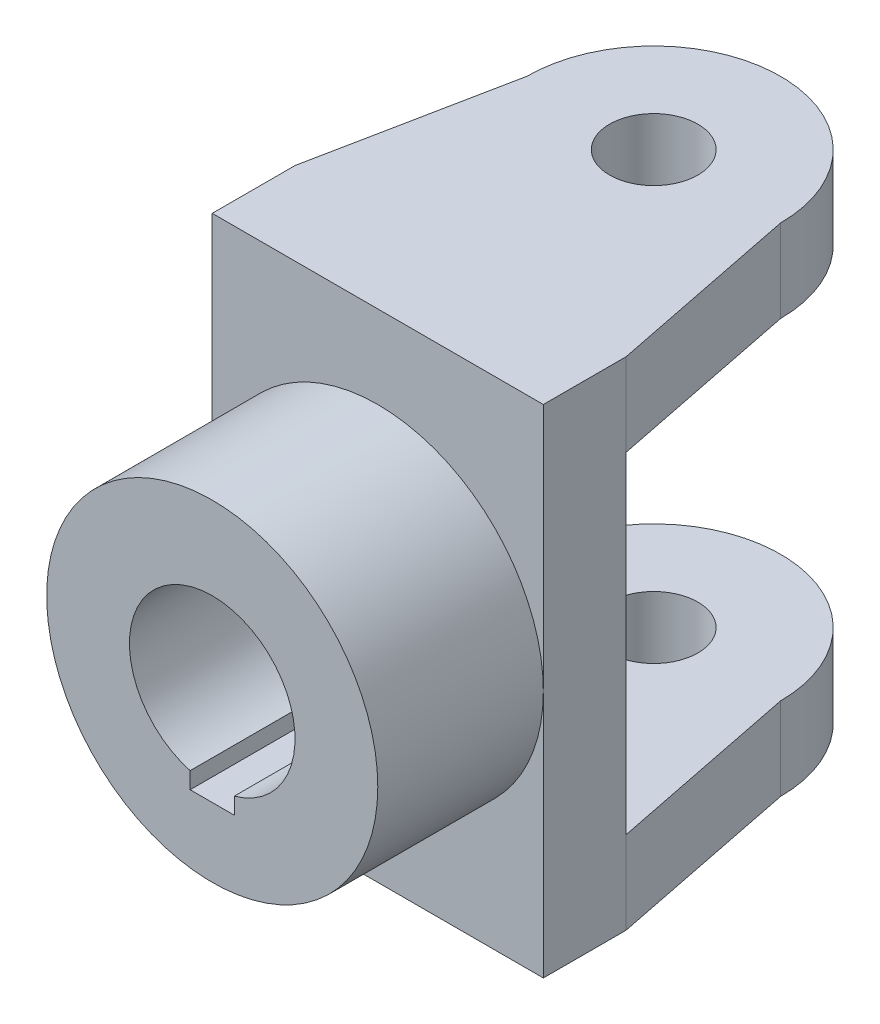
from build123d import *

# Parameters (mm, degrees)
SKETCH1_W           = 60
SKETCH1_H           = 90
BOSS_EXTRUDE1_DEPTH = 15
SKETCH2_R           = 8
BOSS_EXTRUDE2_DEPTH = 15
SKETCH3_R           = 30
BOSS_EXTRUDE3_DEPTH = 30


with BuildPart() as part:
    # Sketch1 → Boss-Extrude1 (new body)
    with BuildSketch(Plane.XY):
        Rectangle(SKETCH1_W, SKETCH1_H)
    extrude(amount=-BOSS_EXTRUDE1_DEPTH)

    # Sketch2 → Boss-Extrude2 (add)
    with BuildSketch(Plane(origin=(0, 45, 0), x_dir=(1, 0, 0), z_dir=(0, 1, 0))):
        with BuildLine():
            Line((-23, 50), (-30, 15))
            Line((-30, 15), (30, 15))
            Line((30, 15), (23, 50))
            ThreePointArc((23, 50), (0, 73), (-23, 50))
        make_face()
        with Locations(Location((0, 50, 0), (0, 0, 270))):
            Circle(SKETCH2_R, mode=Mode.SUBTRACT)
    boss_extrude2 = extrude(amount=-BOSS_EXTRUDE2_DEPTH)

    # Mirror1: Boss-Extrude2 across plane
    add(boss_extrude2.mirror(Plane.ZX))

    # Sketch3 → Boss-Extrude3 (add)
    with BuildSketch(Plane.XY):
        Circle(SKETCH3_R)
        with BuildLine():
            Line((-4, -14.456832295), (-4, -17.456832295))
            Line((-4, -17.456832295), (4, -17.456832295))
            Line((4, -17.456832295), (4, -14.456832295))
            ThreePointArc((4, -14.456832295), (0, 15), (-4, -14.456832295))
        make_face(mode=Mode.SUBTRACT)
    extrude(amount=BOSS_EXTRUDE3_DEPTH)


solid = part.part
